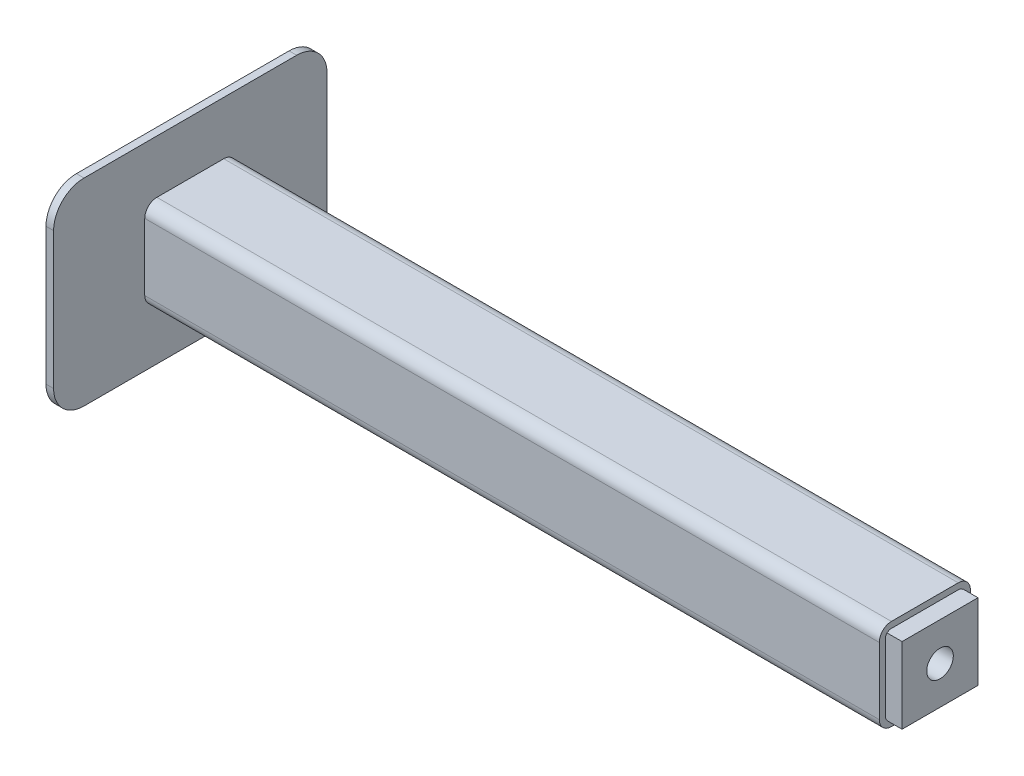
from build123d import *

# Parameters (mm, degrees)
GB_T6728_2002_60_X_60_X_4_1_DEPTH = 483.5
EXTRUDE_1_DEPTH                   = 5
EXTRUDE_2_DEPTH                   = 10
EXTRUDE_2_DEPTH_BACK              = 15
SKETCH_6_W                        = 50
SKETCH_6_H                        = 50


with BuildPart() as part:
    # Sketch1 → 冷弯空心方管gb∕t6728-2002 60 X 60 X 4(1) (new body)
    with BuildSketch(Plane.YZ):
        with BuildLine():
            Line((-22, -30), (22, -30))
            ThreePointArc((22, -30), (27.656854249, -27.656854249), (30, -22))
            Line((30, -22), (30, 22))
            ThreePointArc((30, 22), (27.656854249, 27.656854249), (22, 30))
            Line((22, 30), (-22, 30))
            ThreePointArc((-22, 30), (-27.656854249, 27.656854249), (-30, 22))
            Line((-30, 22), (-30, -22))
            ThreePointArc((-30, -22), (-27.656854249, -27.656854249), (-22, -30))
        make_face()
        with BuildLine():
            Line((-22, -26), (22, -26))
            ThreePointArc((22, -26), (24.828427125, -24.828427125), (26, -22))
            Line((26, -22), (26, 22))
            ThreePointArc((26, 22), (24.828427125, 24.828427125), (22, 26))
            Line((22, 26), (-22, 26))
            ThreePointArc((-22, 26), (-24.828427125, 24.828427125), (-26, 22))
            Line((-26, 22), (-26, -22))
            ThreePointArc((-26, -22), (-24.828427125, -24.828427125), (-22, -26))
        make_face(mode=Mode.SUBTRACT)
    extrude(amount=GB_T6728_2002_60_X_60_X_4_1_DEPTH)


with BuildPart() as body_2:
    # 草图3 → 凸台-拉伸1 (new body)
    with BuildSketch(Plane.ZY):
        with BuildLine():
            Line((-70, 65), (70, 65))
            ThreePointArc((70, 65), (84.142135624, 59.142135624), (90, 45))
            Line((90, 45), (90, -45))
            ThreePointArc((90, -45), (84.142135624, -59.142135624), (70, -65))
            Line((70, -65), (-70, -65))
            ThreePointArc((-70, -65), (-84.142135624, -59.142135624), (-90, -45))
            Line((-90, -45), (-90, 45))
            ThreePointArc((-90, 45), (-84.142135624, 59.142135624), (-70, 65))
        make_face()
    extrude(amount=EXTRUDE_1_DEPTH)


with BuildPart() as body_3:
    # 草图6 → 凸台-拉伸2 (new, two sides: drawn at the far end of the back side and taken through both)
    with BuildSketch(Plane(origin=(483.5, 0, 0), x_dir=(0, 0, -1), z_dir=(1, 0, 0)).offset(-EXTRUDE_2_DEPTH_BACK)):
        Rectangle(SKETCH_6_W, SKETCH_6_H)
    extrude(amount=EXTRUDE_2_DEPTH + EXTRUDE_2_DEPTH_BACK)

    # 草图8 → M20 螺纹孔1 (revolve, cut)
    with BuildSketch(Plane(origin=(493.5, 0, 0), x_dir=(0, 0, -1), z_dir=(0, 1, 0))):
        Polygon((0, 0), (0, 57.757530416), (8.75, 52.5), (8.75, 0), align=None)
    revolve(axis=Axis((499.85, 0, 0), (-1, 0, 0)), mode=Mode.SUBTRACT)


solid = Compound([part.part, body_2.part, body_3.part])
